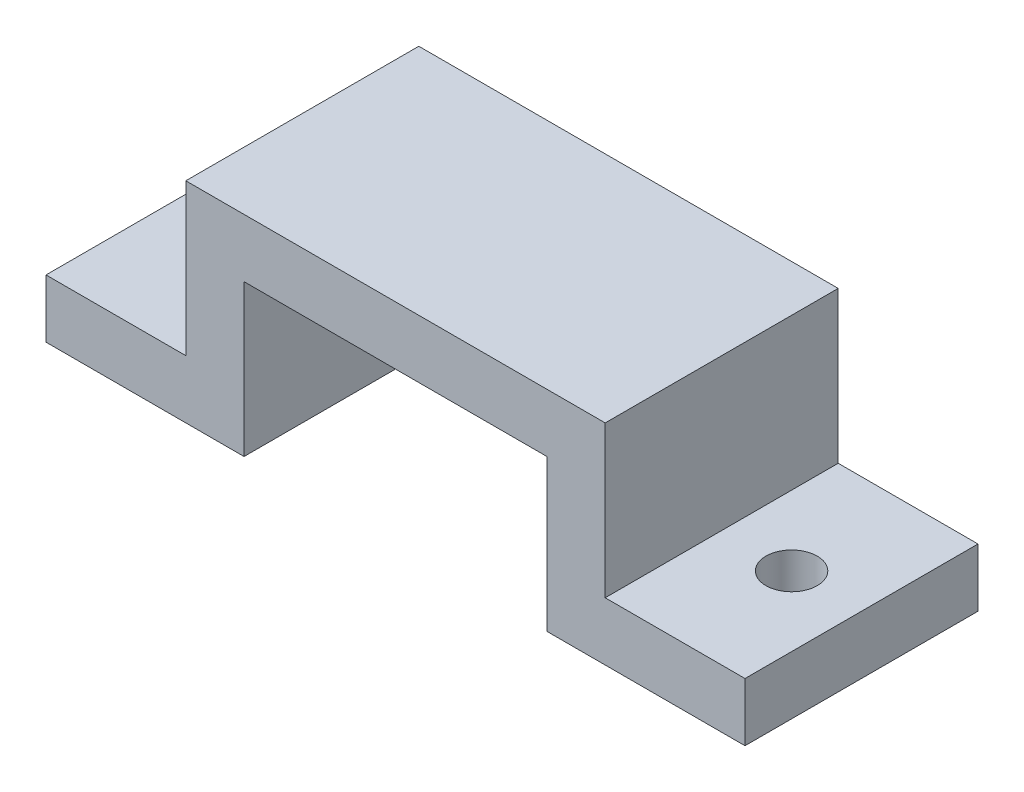
from build123d import *

# Parameters (mm, degrees)
EXTRUDE_1_DEPTH     = 10
SKETCH_2_R          = 2.2
CUT_EXTRUDE_1_DEPTH = 10


with BuildPart() as part:
    # 草图1 → 凸台-拉伸1 (new, symmetric)
    with BuildSketch(Plane.XY):
        Polygon((0, 0), (17, 0), (17, 13), (43, 13), (43, 0), (60, 0), (60, 5), (48, 5), (48, 18), (12, 18), (12, 5), (0, 5), align=None)
    extrude(amount=EXTRUDE_1_DEPTH, both=True)

    # 草图2 → 切除-拉伸1 (cut)
    with BuildSketch(Plane(origin=(0, 5, 0), x_dir=(1, 0, 0), z_dir=(0, 1, 0))):
        with Locations(Location((6, 0, 0), (0, 0, 180))):
            Circle(SKETCH_2_R)
        with Locations(Location((54, 0, 0), (0, 0, 180))):
            Circle(SKETCH_2_R)
    extrude(amount=-CUT_EXTRUDE_1_DEPTH, mode=Mode.SUBTRACT)


solid = part.part
